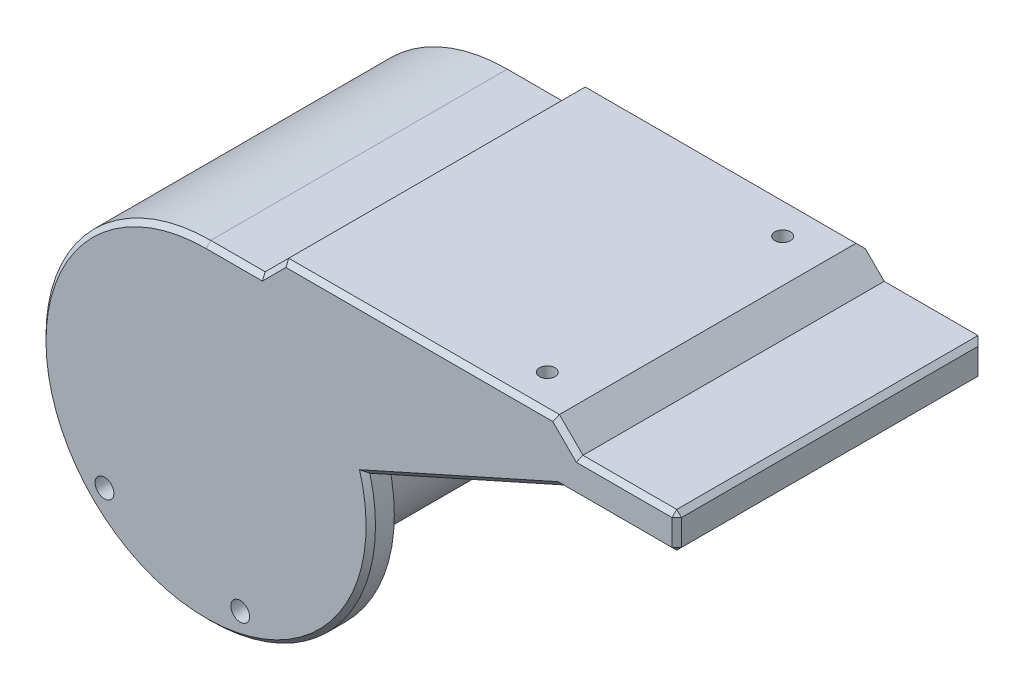
from build123d import *

# Parameters (mm, degrees)
SKETCH_1_R                  = 52
EXTRUDE_1_DEPTH             = 55
SKETCH_2_R                  = 70
EXTRUDE_2_DEPTH             = 10
EXTRUDE_START               = 110
EXTRUDE_3_DEPTH             = 110
EXTRUDE_4_REACH             = 120.427
EXTRUDE_4_DIRECTION_2_REACH = 120.427
SKETCH_5_R                  = 4
CUT_EXTRUDE_1_DEPTH         = 229
SKETCH_6_R                  = 3.3
CUT_EXTRUDE_2_DEPTH         = 68
CUT_EXTRUDE_START           = -30
SKETCH_8_R                  = 8
CUT_EXTRUDE_4_DEPTH         = 168
CHAMFER_1_SIZE              = 2


with BuildPart() as part:
    # 草图1 → 凸台-拉伸1 (new, symmetric)
    with BuildSketch(Plane.XY):
        Circle(SKETCH_1_R)
    extrude(amount=EXTRUDE_1_DEPTH, both=True)

    # 草图2 → 凸台-拉伸2 (add)
    with BuildSketch(Plane.XY.offset(55)):
        Circle(SKETCH_2_R)
    extrude(amount=EXTRUDE_2_DEPTH)

    # 镜向1: part across plane


with BuildPart() as part_1:
    add(part.part)
    add(part.part.mirror(Plane.XY))

    # 草图3 → 凸台-拉伸3 (add)
    with BuildSketch(Plane.XY.offset(-55).offset(EXTRUDE_START)):
        with BuildLine():
            ThreePointArc((67.61480784, 18.117333157), (-18.117333157, 67.61480784), (-67.61480784, -18.117333157))
            Line((-67.61480784, -18.117333157), (-50.228142967, -13.458590345))
            ThreePointArc((-50.228142967, -13.458590345), (-13.458590345, 50.228142967), (50.228142967, 13.458590345))
            Line((50.228142967, 13.458590345), (67.61480784, 18.117333157))
        make_face()
    extrude(amount=-EXTRUDE_3_DEPTH)

    # 凸台-拉伸4: up to this face of the body (flat: up to its plane)
    extrude_4_end = Plane(part_1.part.faces().sort_by_distance((0, 0, 65))[0])
    # 草图4 → 凸台-拉伸4 (add, up to the picked face)
    with BuildSketch(Plane.XY, mode=Mode.PRIVATE) as extrude_4_sk1:
        with BuildLine():
            Line((23.122839281, 70), (0, 70))
            ThreePointArc((0, 70), (42.613300031, 55.53473382), (67.61480784, 18.117333157))
            Line((67.61480784, 18.117333157), (150, 55))
            Line((150, 55), (200, 55))
            Line((200, 55), (200, 70))
            Line((200, 70), (158.152049004, 70))
            Line((158.152049004, 70), (23.122839281, 70))
        make_face()
    extrude_4_tool1 = split(extrude(extrude_4_sk1.sketch, amount=EXTRUDE_4_REACH, mode=Mode.PRIVATE), bisect_by=extrude_4_end, keep=Keep.BOTH, mode=Mode.PRIVATE)
    # 草图4 → 凸台-拉伸4 (add, up to the picked face)
    with BuildSketch(Plane.XY, mode=Mode.PRIVATE) as extrude_4_sk2:
        Polygon((33.122839281, 80), (23.122839281, 70), (158.152049004, 70), (148.152049004, 80), align=None)
    extrude_4_tool2 = split(extrude(extrude_4_sk2.sketch, amount=EXTRUDE_4_REACH, mode=Mode.PRIVATE), bisect_by=extrude_4_end, keep=Keep.BOTH, mode=Mode.PRIVATE)
    add(extrude_4_tool1.solids().sort_by(Axis((103.613169, 54.432495, 0), (0, 0, 1)))[0])
    add(extrude_4_tool2.solids().sort_by(Axis((90.637444, 74.866698, 0), (0, 0, 1)))[0])

    # 凸台-拉伸4 direction 2: up to this face of the body (flat: up to its plane)
    extrude_4_direction_2_end = Plane(part_1.part.faces().sort_by_distance((0, 0, -65))[0])
    # 草图4 → 凸台-拉伸4 direction 2 (add, up to the picked face)
    with BuildSketch(Plane.XY, mode=Mode.PRIVATE) as extrude_4_direction_2_sk1:
        with BuildLine():
            Line((23.122839281, 70), (0, 70))
            ThreePointArc((0, 70), (42.613300031, 55.53473382), (67.61480784, 18.117333157))
            Line((67.61480784, 18.117333157), (150, 55))
            Line((150, 55), (200, 55))
            Line((200, 55), (200, 70))
            Line((200, 70), (158.152049004, 70))
            Line((158.152049004, 70), (23.122839281, 70))
        make_face()
    extrude_4_direction_2_tool1 = split(extrude(extrude_4_direction_2_sk1.sketch, amount=-EXTRUDE_4_DIRECTION_2_REACH, mode=Mode.PRIVATE), bisect_by=extrude_4_direction_2_end, keep=Keep.BOTH, mode=Mode.PRIVATE)
    # 草图4 → 凸台-拉伸4 direction 2 (add, up to the picked face)
    with BuildSketch(Plane.XY, mode=Mode.PRIVATE) as extrude_4_direction_2_sk2:
        Polygon((33.122839281, 80), (23.122839281, 70), (158.152049004, 70), (148.152049004, 80), align=None)
    extrude_4_direction_2_tool2 = split(extrude(extrude_4_direction_2_sk2.sketch, amount=-EXTRUDE_4_DIRECTION_2_REACH, mode=Mode.PRIVATE), bisect_by=extrude_4_direction_2_end, keep=Keep.BOTH, mode=Mode.PRIVATE)
    add(extrude_4_direction_2_tool1.solids().sort_by(Axis((103.613169, 54.432495, 0), (0, 0, -1)))[0])
    add(extrude_4_direction_2_tool2.solids().sort_by(Axis((90.637444, 74.866698, 0), (0, 0, -1)))[0])

    # 草图5 → 切除-拉伸1 (cut)
    with BuildSketch(Plane.XY.offset(65)):
        with Locations(Location((-43.16038802, -41.679502228, 0), (0, 0, 180))):
            Circle(SKETCH_5_R)
        with Locations(Location((14.515313736, -58.217743577, 0), (0, 0, 180))):
            Circle(SKETCH_5_R)
    extrude(amount=-CUT_EXTRUDE_1_DEPTH, mode=Mode.SUBTRACT)

    # 草图6 → 切除-拉伸2 (cut)
    with BuildSketch(Plane(origin=(0, 80, 0), x_dir=(1, 0, 0), z_dir=(0, 1, 0))):
        with Locations(Location((130, 50, 0), (0, 0, 270))):
            Circle(SKETCH_6_R)
        with Locations(Location((130, -50, 0), (0, 0, 270))):
            Circle(SKETCH_6_R)
    extrude(amount=-CUT_EXTRUDE_2_DEPTH, mode=Mode.SUBTRACT)

    # 草图8 → 切除-拉伸4 (cut)
    with BuildSketch(Plane(origin=(0, 80, 0), x_dir=(1, 0, 0), z_dir=(0, 1, 0)).offset(CUT_EXTRUDE_START)):
        with Locations(Location((130, 50, 0), (0, 0, 270))):
            Circle(SKETCH_8_R)
        with Locations(Location((130, -50, 0), (0, 0, 270))):
            Circle(SKETCH_8_R)
    extrude(amount=-CUT_EXTRUDE_4_DEPTH, mode=Mode.SUBTRACT)

    # 倒角1
    chamfer_1_edges = [part_1.edges().sort_by_distance(p)[0] for p in [
        (-42.613300031, -55.53473382, -65),
        (-42.613300031, -55.53473382, 65),
        (11.561419641, 70, 65),
        (28.122839281, 75, 65),
        (90.637444143, 80, 65),
        (153.152049004, 75, 65),
        (179.076024502, 70, 65),
        (200, 70, 0),
        (200, 62.5, 65),
        (200, 55, 0),
        (175, 55, 65),
        (108.80740392, 36.558666579, 65),
        (108.80740392, 36.558666579, -65),
        (11.561419641, 70, -65),
        (28.122839281, 75, -65),
        (90.637444143, 80, -65),
        (200, 62.5, -65),
        (175, 55, -65),
    ]]
    chamfer(chamfer_1_edges, length=CHAMFER_1_SIZE)


solid = part_1.part
